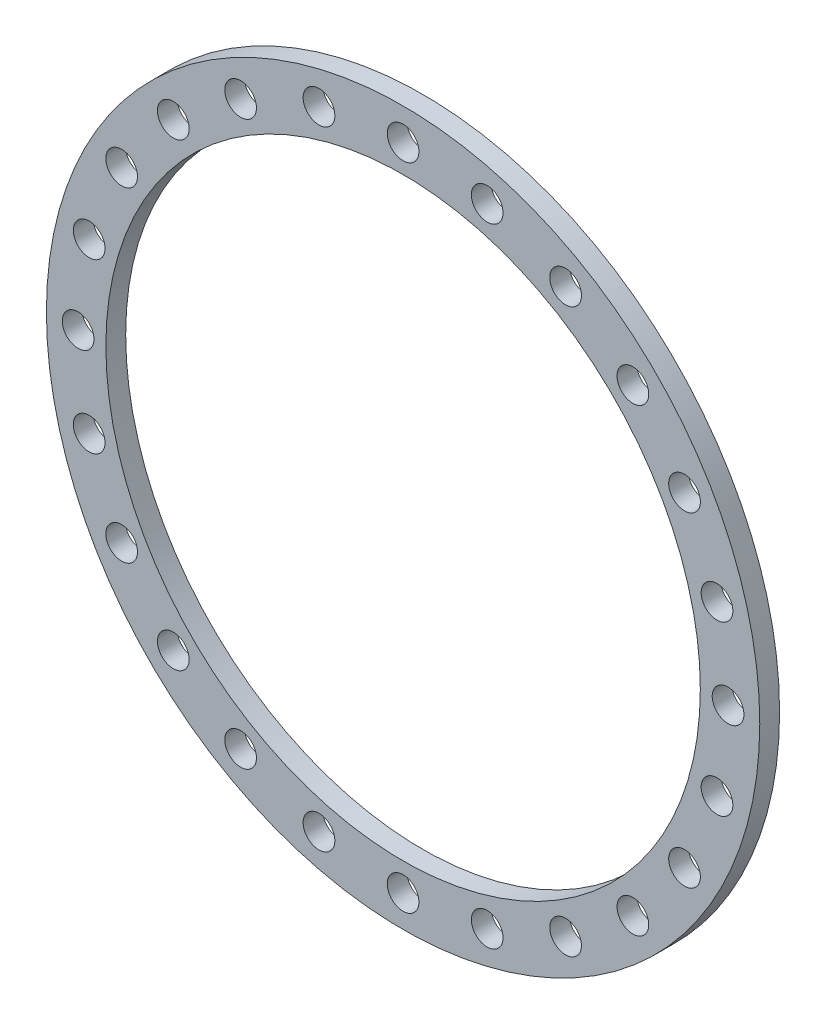
from build123d import *

# Parameters (mm, degrees)
SKETCH_1_R          = 450
EXTRUDE_1_DEPTH     = 25
SKETCH_2_R          = 20
CUT_EXTRUDE_1_DEPTH = 34
SKETCH_3_R          = 375
CUT_EXTRUDE_2_DEPTH = 420


with BuildPart() as part:
    # 草图1 → 凸台-拉伸1 (new body)
    with BuildSketch(Plane.XY):
        Circle(SKETCH_1_R)
    extrude(amount=EXTRUDE_1_DEPTH)

    # 草图2 → 切除-拉伸1 (cut)
    with BuildSketch(Plane.XY.offset(25)):
        with Locations((0, 410)):
            Circle(SKETCH_2_R)
        with Locations((106.115808492, 396.029588779)):
            Circle(SKETCH_2_R)
        with Locations((205, 355.070415552)):
            Circle(SKETCH_2_R)
        with Locations((289.913780286, 289.913780286)):
            Circle(SKETCH_2_R)
        with Locations((355.070415552, 205)):
            Circle(SKETCH_2_R)
        with Locations((396.029588779, 106.115808492)):
            Circle(SKETCH_2_R)
        with Locations((410, 0)):
            Circle(SKETCH_2_R)
        with Locations((396.029588779, -106.115808492)):
            Circle(SKETCH_2_R)
        with Locations((355.070415552, -205)):
            Circle(SKETCH_2_R)
        with Locations((289.913780286, -289.913780286)):
            Circle(SKETCH_2_R)
        with Locations((205, -355.070415552)):
            Circle(SKETCH_2_R)
        with Locations((106.115808492, -396.029588779)):
            Circle(SKETCH_2_R)
        with Locations((0, -410)):
            Circle(SKETCH_2_R)
        with Locations((-106.115808492, -396.029588779)):
            Circle(SKETCH_2_R)
        with Locations((-205, -355.070415552)):
            Circle(SKETCH_2_R)
        with Locations((-289.913780286, -289.913780286)):
            Circle(SKETCH_2_R)
        with Locations((-355.070415552, -205)):
            Circle(SKETCH_2_R)
        with Locations((-396.029588779, -106.115808492)):
            Circle(SKETCH_2_R)
        with Locations((-410, 0)):
            Circle(SKETCH_2_R)
        with Locations((-396.029588779, 106.115808492)):
            Circle(SKETCH_2_R)
        with Locations((-355.070415552, 205)):
            Circle(SKETCH_2_R)
        with Locations((-289.913780286, 289.913780286)):
            Circle(SKETCH_2_R)
        with Locations((-205, 355.070415552)):
            Circle(SKETCH_2_R)
        with Locations((-106.115808492, 396.029588779)):
            Circle(SKETCH_2_R)
    extrude(amount=-CUT_EXTRUDE_1_DEPTH, mode=Mode.SUBTRACT)

    # 草图3 → 切除-拉伸2 (cut)
    with BuildSketch(Plane.XY.offset(25)):
        Circle(SKETCH_3_R)
    extrude(amount=-CUT_EXTRUDE_2_DEPTH, mode=Mode.SUBTRACT)


solid = part.part
